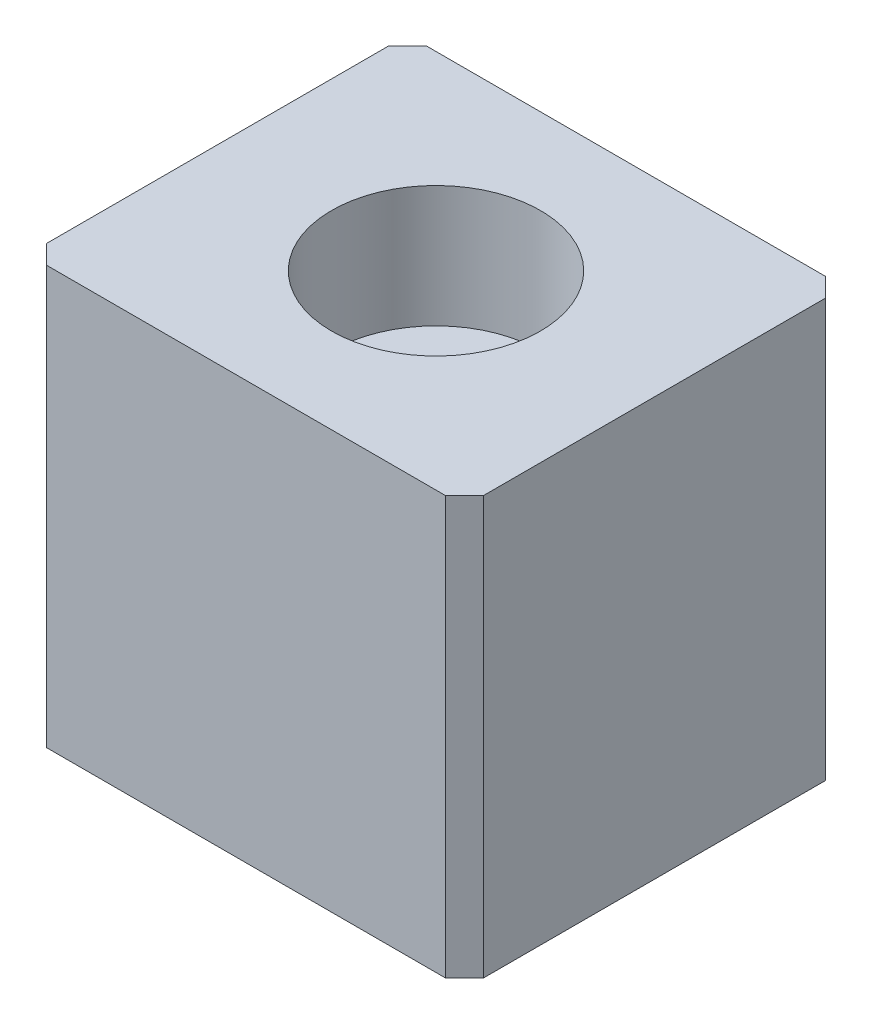
SolidWorks part; units mm, degrees
material "AL6061"
ref_plane "前视基准面" through (0, 0, 0) normal (0, 0, 1) x (1, 0, 0)
ref_plane "上视基准面" through (0, 0, 0) normal (0, 1, 0) x (1, 0, 0)
ref_plane "右视基准面" through (0, 0, 0) normal (1, 0, 0) x (0, 0, -1)
sketch "草图1" plane through (0, 0, 0) normal (0, 1, 0) x (1, 0, 0)
  line L0 (0, 10) -> (0, 0) construction
  line L1 (-11.5, 10) -> (11.5, 10)
  line L2 (-11.5, 10) -> (-11.5, -10)
  line L3 (-11.5, -10) -> (11.5, -10)
  line L4 (11.5, 10) -> (11.5, -10)
  line L5 (0, 0) -> (11.5, 0) construction
  dimension "D1" = 23
  dimension "D2" = 20
extrude "凸台-拉伸1" add sketch "草图1" along normal mid plane 22
hole_wizard "M6 六角凹头螺钉的柱形沉头孔1" positions "草图3" profile "草图2" counterbore size "M6" standard "Iso" end condition through all
sketch "草图3" plane through (0, 11, 0) normal (0, 1, 0) x (1, 0, 0)
  point P0 (0, 0)
sketch "草图2" plane through (0, 11, 0) normal (1, 0, 0) x (0, 0, 1)
  line L0 (0, 0) -> (0, 22)
  line L1 (0, 22) -> (3.3, 22)
  line L3 (3.3, 22) -> (3.3, 6.4)
  line L4 (3.3, 6.4) -> (5.5, 6.4)
  line L5 (5.5, 6.4) -> (5.5, 0)
  line L7 (5.5, 0) -> (0, 0)
  line L11 (0, -6.35) -> (0, 107.95) construction
  dimension "通孔孔直径" = 6.6
  dimension "通孔孔深度" = 22
  dimension "柱形沉头孔直径" = 11
  dimension "柱形沉头孔深度" = 6.4
chamfer "倒角1" distance 1 angle 45 4 edges at (11.5, 0, 10) (-11.5, 0, 10) (11.5, 0, -10) (-11.5, 0, -10)
